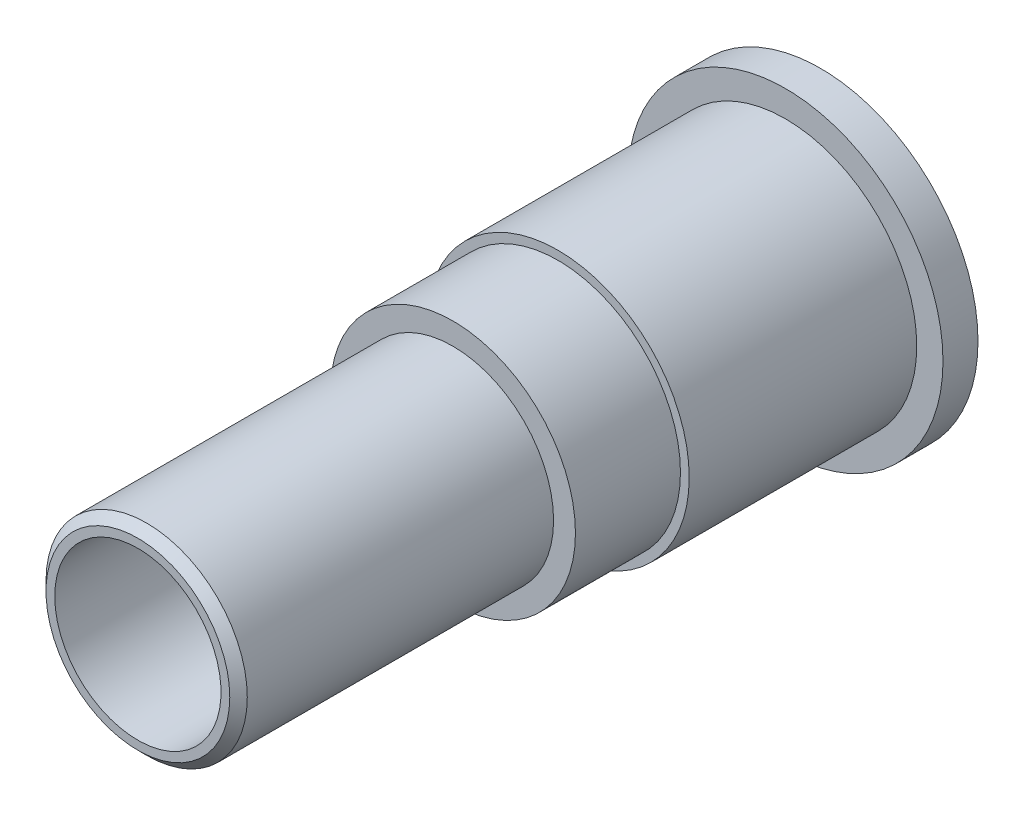
from build123d import *

# Parameters (mm, degrees)
SKETCH1_R           = 9
BOSS_EXTRUDE1_DEPTH = 2
SKETCH2_R           = 7.5
BOSS_EXTRUDE2_DEPTH = 13
SKETCH3_R           = 7
BOSS_EXTRUDE3_DEPTH = 6
SKETCH5_R           = 5.75
BOSS_EXTRUDE4_DEPTH = 18
SKETCH4_R           = 4.75
CUT_EXTRUDE1_DEPTH  = 42.024382994
CHAMFER1_SIZE       = 0.5
CHAMFER2_SIZE       = 0.3
CHAMFER2_SIZE2      = 10


with BuildPart() as part:
    # Sketch1 → Boss-Extrude1 (new body)
    with BuildSketch(Plane.XY):
        Circle(SKETCH1_R)
    extrude(amount=BOSS_EXTRUDE1_DEPTH)

    # Sketch2 → Boss-Extrude2 (add)
    with BuildSketch(Plane.XY.offset(2)):
        with Locations(Location((0, 0, 0), (0, 0, 180))):
            Circle(SKETCH2_R)
    extrude(amount=BOSS_EXTRUDE2_DEPTH)

    # Sketch3 → Boss-Extrude3 (add)
    with BuildSketch(Plane.XY.offset(15)):
        Circle(SKETCH3_R)
    extrude(amount=BOSS_EXTRUDE3_DEPTH)

    # Sketch5 → Boss-Extrude4 (add)
    with BuildSketch(Plane.XY.offset(21)):
        Circle(SKETCH5_R)
    extrude(amount=BOSS_EXTRUDE4_DEPTH)

    # Sketch4 → Cut-Extrude1 (cut, through all)
    with BuildSketch(Plane(origin=(0, 0, 0), x_dir=(-1, 0, 0), z_dir=(0, 0, -1))):
        Circle(SKETCH4_R)
    extrude(amount=-CUT_EXTRUDE1_DEPTH, mode=Mode.SUBTRACT)

    # Chamfer1
    chamfer1_edges = [part.edges().sort_by_distance(p)[0] for p in [
        (-5.75, 0, 39),
    ]]
    chamfer(chamfer1_edges, length=CHAMFER1_SIZE)

    # Chamfer2
    chamfer2_edges = [part.edges().sort_by_distance(p)[0] for p in [
        (4.75, 0, 0),
    ]]
    chamfer2_side = [part.faces().sort_by_distance(p)[0] for p in [
        (-8.745441559, 0, 0),
    ]]
    chamfer(chamfer2_edges, length=CHAMFER2_SIZE, length2=CHAMFER2_SIZE2, reference=chamfer2_side[0])


solid = part.part
